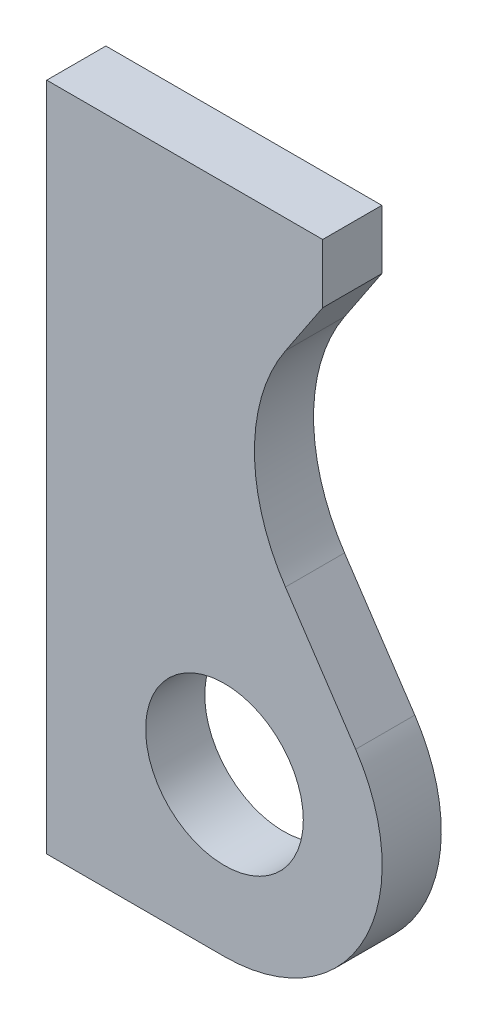
SolidWorks part; units mm, degrees
ref_plane "前视基准面" through (0, 0, 0) normal (0, 0, 1) x (1, 0, 0)
ref_plane "上视基准面" through (0, 0, 0) normal (0, 1, 0) x (1, 0, 0)
ref_plane "右视基准面" through (0, 0, 0) normal (1, 0, 0) x (0, 0, -1)
sketch "草图1" plane through (0, 0, 0) normal (0, 0, 1) x (1, 0, 0)
  line L0 (0, 0) -> (70, 0)
  line L1 (70, 0) -> (70, -15)
  line L4 (50, -45) -> (70, -15)
  line L5 (50, -45) -> (50, -65.2661)
  line L6 (0, 0) -> (0, -170)
  line L7 (0, -170) -> (45.0819, -170)
  line L8 (78.3639, -107.812) -> (50, -65.2661)
  arc A0 (78.3639, -107.812) -> (45.0819, -170) centre (45.0819, -130) cw
  circle A1 centre (45.0819, -130) radius 20
  dimension "D1" = 40
extrude "凸台-拉伸1" add sketch "草图1" along normal blind 12
sketch "草图3" plane through (0, 0, 12) normal (0, 0, 1) x (1, 0, 0)
  line L0 (50, -55.133) -> (99.4661, -55.133)
  line L4 (50, -65.2661) -> (50, -45) construction
  line L5 (60.5436, -29.1847) -> (50, -45)
  line L6 (50, -45) -> (50, -65.2661)
  line L7 (50, -65.2661) -> (60.5436, -81.0814)
  circle A0 centre (99.4661, -55.133) radius 46.7791
  line M4 (78.3639, -107.812) -> (50, -65.2661)
  line M5 (50, -65.2661) -> (50, -45)
  line M6 (50, -45) -> (70, -15)
extrude "凸台-拉伸2" add sketch "草图3" against normal blind 10 contours A0 L0 M6 M5 | A0 L0 M5 M4
sketch "草图4" plane through (0, 0, 2) normal (0, 0, -1) x (-1, 0, 0)
  line L6 (-60.5436, -81.0814) -> (-50, -65.2661)
  line L7 (-50, -65.2661) -> (-50, -45)
  line L8 (-50, -45) -> (-60.5436, -29.1847)
  line L9 (-60.5436, -81.0814) -> (-50, -65.2661)
  line L10 (-50, -65.2661) -> (-50, -45)
  line L11 (-50, -45) -> (-60.5436, -29.1847)
  arc A2 (-60.5436, -81.0814) -> (-60.5436, -29.1847) centre (-99.4661, -55.133) ccw
  arc A3 (-60.5436, -81.0814) -> (-60.5436, -29.1847) centre (-99.4661, -55.133) ccw
  dimension "D1" = 0
extrude "凸台-拉伸3" add sketch "草图4" along normal blind 2
sketch "草图5" plane through (0, 0, 12) normal (0, 0, 1) x (1, 0, 0)
  line L12 (0, 0) -> (0, -170)
  line L13 (0, -170) -> (45.0819, -170)
  line L14 (78.3639, -107.812) -> (60.5436, -81.0814)
  line L15 (60.5436, -29.1847) -> (70, -15)
  line L16 (70, -15) -> (70, 0)
  line L17 (70, 0) -> (0, 0)
  line L18 (0, 0) -> (0, -170)
  line L19 (0, -170) -> (45.0819, -170)
  line L20 (78.3639, -107.812) -> (60.5436, -81.0814)
  line L21 (60.5436, -29.1847) -> (70, -15)
  line L22 (70, -15) -> (70, 0)
  line L23 (70, 0) -> (0, 0)
  arc A4 (45.0819, -170) -> (78.3639, -107.812) centre (45.0819, -130) ccw
  arc A5 (60.5436, -29.1847) -> (60.5436, -81.0814) centre (99.4661, -55.133) ccw
  arc A6 (45.0819, -170) -> (78.3639, -107.812) centre (45.0819, -130) ccw
  arc A7 (60.5436, -29.1847) -> (60.5436, -81.0814) centre (99.4661, -55.133) ccw
  circle A8 centre (45.0819, -130) radius 20
  circle A9 centre (45.0819, -130) radius 20
  dimension "D1" = 0
  dimension "D2" = 0
extrude "凸台-拉伸4" add sketch "草图5" along normal blind 3
